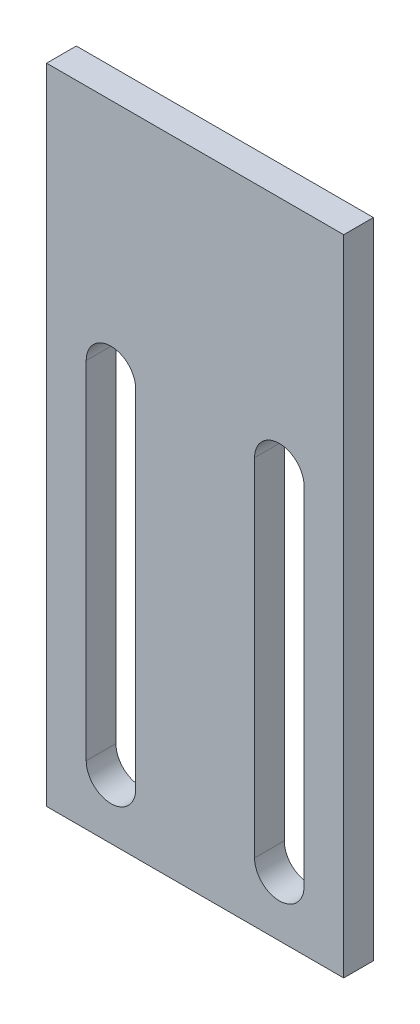
SolidWorks part; units mm, degrees
ref_plane "前视基准面" through (0, 0, 0) normal (0, 0, 1) x (1, 0, 0)
ref_plane "上视基准面" through (0, 0, 0) normal (0, 1, 0) x (1, 0, 0)
ref_plane "右视基准面" through (0, 0, 0) normal (1, 0, 0) x (0, 0, -1)
sketch "草图1" plane through (0, 0, 0) normal (0, 0, 1) x (1, 0, 0)
  line L1 (-15, -32.5) -> (15, -32.5)
  line L2 (-15, -32.5) -> (-15, 32.5)
  line L3 (-15, 32.5) -> (15, 32.5)
  line L4 (15, -32.5) -> (15, 32.5)
  line L5 (-15, -32.5) -> (15, 32.5) construction
  line L6 (-15, 32.5) -> (15, -32.5) construction
  point P0 (0, 0)
  dimension "D1" = 30
  dimension "D2" = 65
extrude "凸台-拉伸1" add sketch "草图1" along normal blind 3
sketch "草图2" plane through (0, 0, 3) normal (0, 0, 1) x (1, 0, 0)
  line L0 (-8.5, -26.5) -> (-8.5, 8.5) construction
  line L1 (-11, -26.5) -> (-11, 8.5)
  line L2 (-6, -26.5) -> (-6, 8.5)
  line L3 (-15, 32.5) -> (-15, -32.5) construction
  line L4 (-15, -32.5) -> (15, -32.5) construction
  arc A0 (-11, -26.5) -> (-6, -26.5) centre (-8.5, -26.5) ccw
  arc A1 (-6, 8.5) -> (-11, 8.5) centre (-8.5, 8.5) ccw
  point P2 (-8.5, -9)
  dimension "D2" = 2.5
  dimension "D1" = 35
  dimension "D3" = 4
  dimension "D4" = 6
extrude "切除-拉伸1" cut sketch "草图2" against normal up to next
mirror "镜向1" about plane through (0, 0, 0) normal (1, 0, 0) of "切除-拉伸1"
